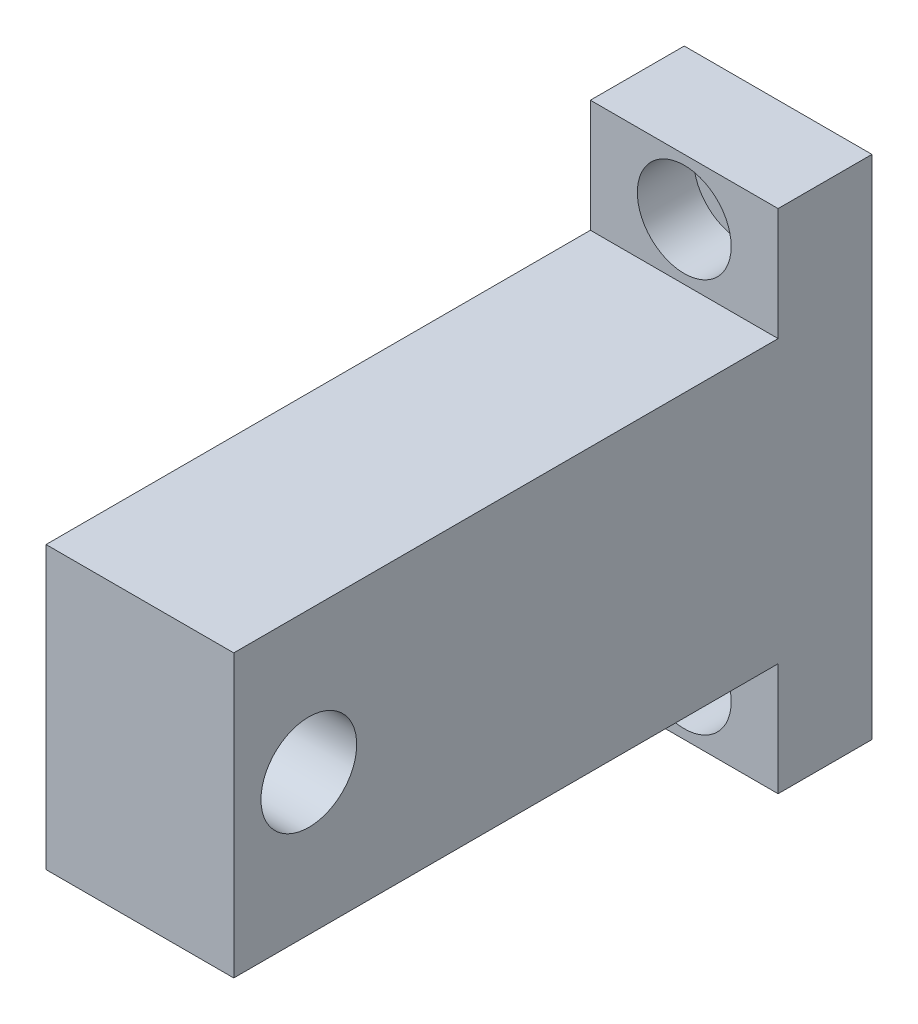
from build123d import *

# Parameters (mm, degrees)
SKETCH1_W                               = 20
SKETCH1_H                               = 54
BOSS_EXTRUDE1_DEPTH                     = 10
SKETCH2_W                               = 20
SKETCH2_H                               = 30
BOSS_EXTRUDE2_DEPTH                     = 58
CBORE_FOR_M6_HEX_HEAD_BOLT1_D           = 6.6
CBORE_FOR_M6_HEX_HEAD_BOLT1_CBORE_D     = 10
CBORE_FOR_M6_HEX_HEAD_BOLT1_CBORE_DEPTH = 6
M12_TAPPED_HOLE1_D                      = 10.2


with BuildPart() as part:
    # Sketch1 → Boss-Extrude1 (new body)
    with BuildSketch(Plane.XY):
        with Locations((-26.388136882, 2.617870722)):
            Rectangle(SKETCH1_W, SKETCH1_H)
    extrude(amount=BOSS_EXTRUDE1_DEPTH)

    # Sketch2 → Boss-Extrude2 (add)
    with BuildSketch(Plane.XY.offset(10)):
        with Locations((-26.388136882, 2.617870722)):
            Rectangle(SKETCH2_W, SKETCH2_H)
    extrude(amount=BOSS_EXTRUDE2_DEPTH)

    # CBORE for M6 Hex Head Bolt1 (through all)
    with Locations(Plane.XY.offset(10)):
        with Locations((-26.388136882, 23.617870722), (-26.388136882, -18.382129278)):
            CounterBoreHole(CBORE_FOR_M6_HEX_HEAD_BOLT1_D / 2, CBORE_FOR_M6_HEX_HEAD_BOLT1_CBORE_D / 2, CBORE_FOR_M6_HEX_HEAD_BOLT1_CBORE_DEPTH)

    # M12 Tapped Hole1 (through all)
    with Locations(Plane.ZY.offset(36.388136882)):
        with Locations((60, 2.617870722)):
            Hole(M12_TAPPED_HOLE1_D / 2)


solid = part.part
